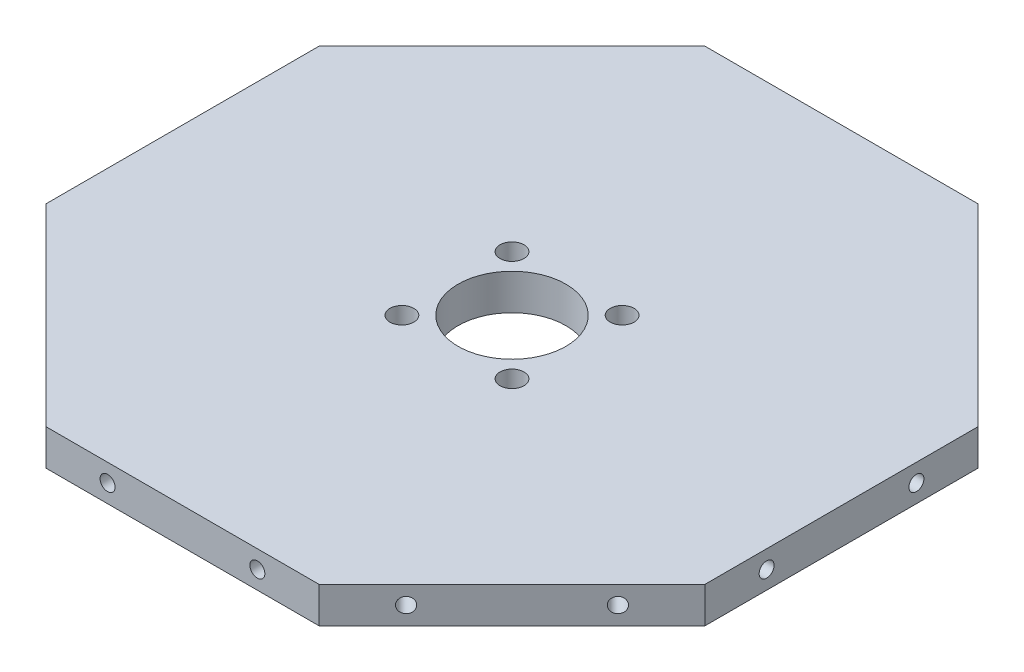
SolidWorks part; units mm, degrees
material "尼龙 101"
ref_plane "前视基准面" through (0, 0, 0) normal (0, 0, 1) x (1, 0, 0)
ref_plane "上视基准面" through (0, 0, 0) normal (0, 1, 0) x (1, 0, 0)
ref_plane "右视基准面" through (0, 0, 0) normal (1, 0, 0) x (0, 0, -1)
sketch "草图1" plane through (0, 0, 0) normal (0, 0, 1) x (1, 0, 0)
  line L0 (0, 0) -> (0, 8.0544) construction
  line L1 (0, 0) -> (18, 0) construction
  line L2 (120, -6) -> (10, -6) construction
  line L3 (0, 0) -> (0, 55) construction
  line L5 (18, 6) -> (18, -6)
  line L6 (18, -6) -> (120, -6)
  line L7 (120, 6) -> (120, -6)
  line L8 (18, 6) -> (120, -6) construction
  line L9 (18, -6) -> (120, 6) construction
  line L12 (120, 6) -> (18, 6)
  point P2 (69, 0)
  dimension "D1" = 18
  dimension "D2" = 120
  dimension "D3" = 12
revolve "旋转1" add sketch "草图1" angle 360 about L3
sketch "草图2" plane through (0, 0, 0) normal (0, 1, 0) x (1, 0, 0)
  line L0 (0, 0) -> (117.3669, 0) construction
  line L1 (117.3669, 0) -> (117.3669, 25) construction
  circle A0 centre (0, 0) radius 120 construction
  dimension "D1" = 25
sketch "草图4" plane through (0, 6, 0) normal (0, 1, 0) x (1, 0, 0)
  line L0 (110, 47.9583) -> (110, -47.9583)
  circle A0 centre (0, 0) radius 120 construction
  circle A1 centre (0, 0) radius 120
  circle M2 centre (0, 0) radius 120
  dimension "D1" = 110
extrude "切除-拉伸1" cut sketch "草图4" against normal blind 83 contours L0 M2
sketch "草图5" plane through (110, 0, 0) normal (1, 0, 0) x (0, 0, -1)
  line L0 (-25, 0) -> (25, 0) construction
  dimension "D1" = 50
hole_wizard "M6x1.0 螺纹孔1" positions "3D草图2" profile "草图6" tap size "M6x1.0" standard "BSI"
sketch3d "3D草图2"
  point P0 (110, 0, 25)
  point P3 (110, 0, -25)
sketch "草图6" plane through (110, 0, 25) normal (0, 1, 0) x (0, 0, -1)
  line L0 (0, 0) -> (0, 13.5022)
  line L1 (0, 13.5022) -> (2.5, 12)
  line L2 (2.5, 12) -> (2.5, 0)
  line L5 (2.5, 0) -> (0, 0)
  line L10 (0, 13.5022) -> (-2.5, 12) construction
  line L11 (0, -6.35) -> (0, 107.95) construction
  dimension "螺纹孔钻头直径" = 5
  dimension "螺纹孔钻头深度" = 12
  dimension "导头角度" = 118
cosmetic thread "孔螺蚊线2" parameters "D1"=12, "D2"=6
cosmetic thread "孔螺蚊线3" parameters "D1"=12, "D2"=6
pattern_circular "阵列(圆周)1" count 8 over 360 about axis through (0, 0, 0) along (0, 1, 0) of "切除-拉伸1", "M6x1.0 螺纹孔1"
cosmetic thread "孔螺蚊线4" parameters "D1"=12, "D2"=6
cosmetic thread "孔螺蚊线5" parameters "D1"=12, "D2"=6
cosmetic thread "孔螺蚊线6" parameters "D1"=12, "D2"=6
cosmetic thread "孔螺蚊线7" parameters "D1"=12, "D2"=6
cosmetic thread "孔螺蚊线8" parameters "D1"=12, "D2"=6
cosmetic thread "孔螺蚊线9" parameters "D1"=12, "D2"=6
cosmetic thread "孔螺蚊线10" parameters "D1"=12, "D2"=6
cosmetic thread "孔螺蚊线11" parameters "D1"=12, "D2"=6
cosmetic thread "孔螺蚊线12" parameters "D1"=12, "D2"=6
cosmetic thread "孔螺蚊线13" parameters "D1"=12, "D2"=6
cosmetic thread "孔螺蚊线14" parameters "D1"=12, "D2"=6
cosmetic thread "孔螺蚊线15" parameters "D1"=12, "D2"=6
cosmetic thread "孔螺蚊线16" parameters "D1"=12, "D2"=6
cosmetic thread "孔螺蚊线17" parameters "D1"=12, "D2"=6
sketch "草图7" plane through (0, 6, 0) normal (0, 1, 0) x (1, 0, 0)
  line L0 (0, 0) -> (18.3848, 18.3848) construction
  line L3 (-110, -45.5635) -> (-110, 45.5635) construction
  circle A0 centre (18.3848, 18.3848) radius 1.65
  dimension "D2" = 3.3
  dimension "D1" = 26
  dimension "D3" = 45
extrude "切除-拉伸2" cut sketch "草图7" against normal blind 30
sketch "草图8" plane through (0, 6, 0) normal (0, 1, 0) x (1, 0, 0)
  circle A0 centre (18.3848, 18.3848) radius 4
  dimension "D1" = 8
extrude "切除-拉伸3" cut sketch "草图8" against normal blind 7
pattern_circular "阵列(圆周)2" count 4 over 360 about axis through (0, 0, 0) along (0, 1, 0) of "切除-拉伸2", "切除-拉伸3"
